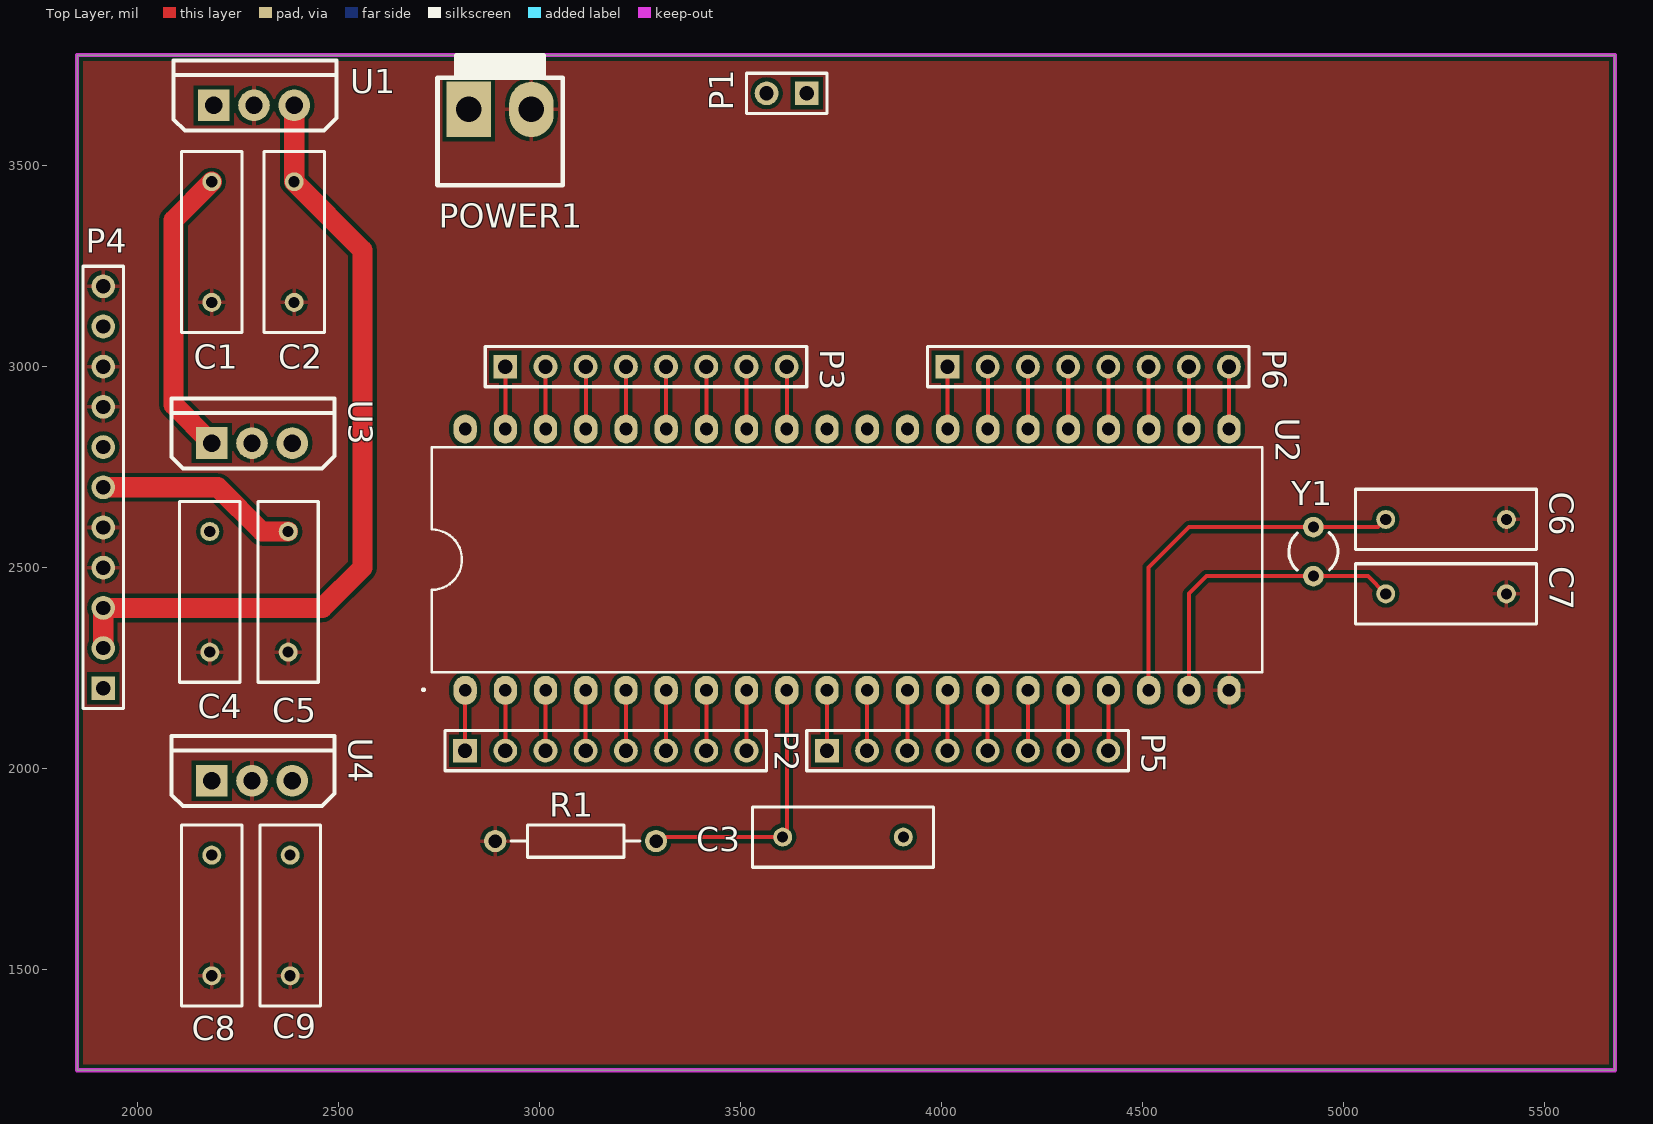
[diagram p0: Top Layer view]
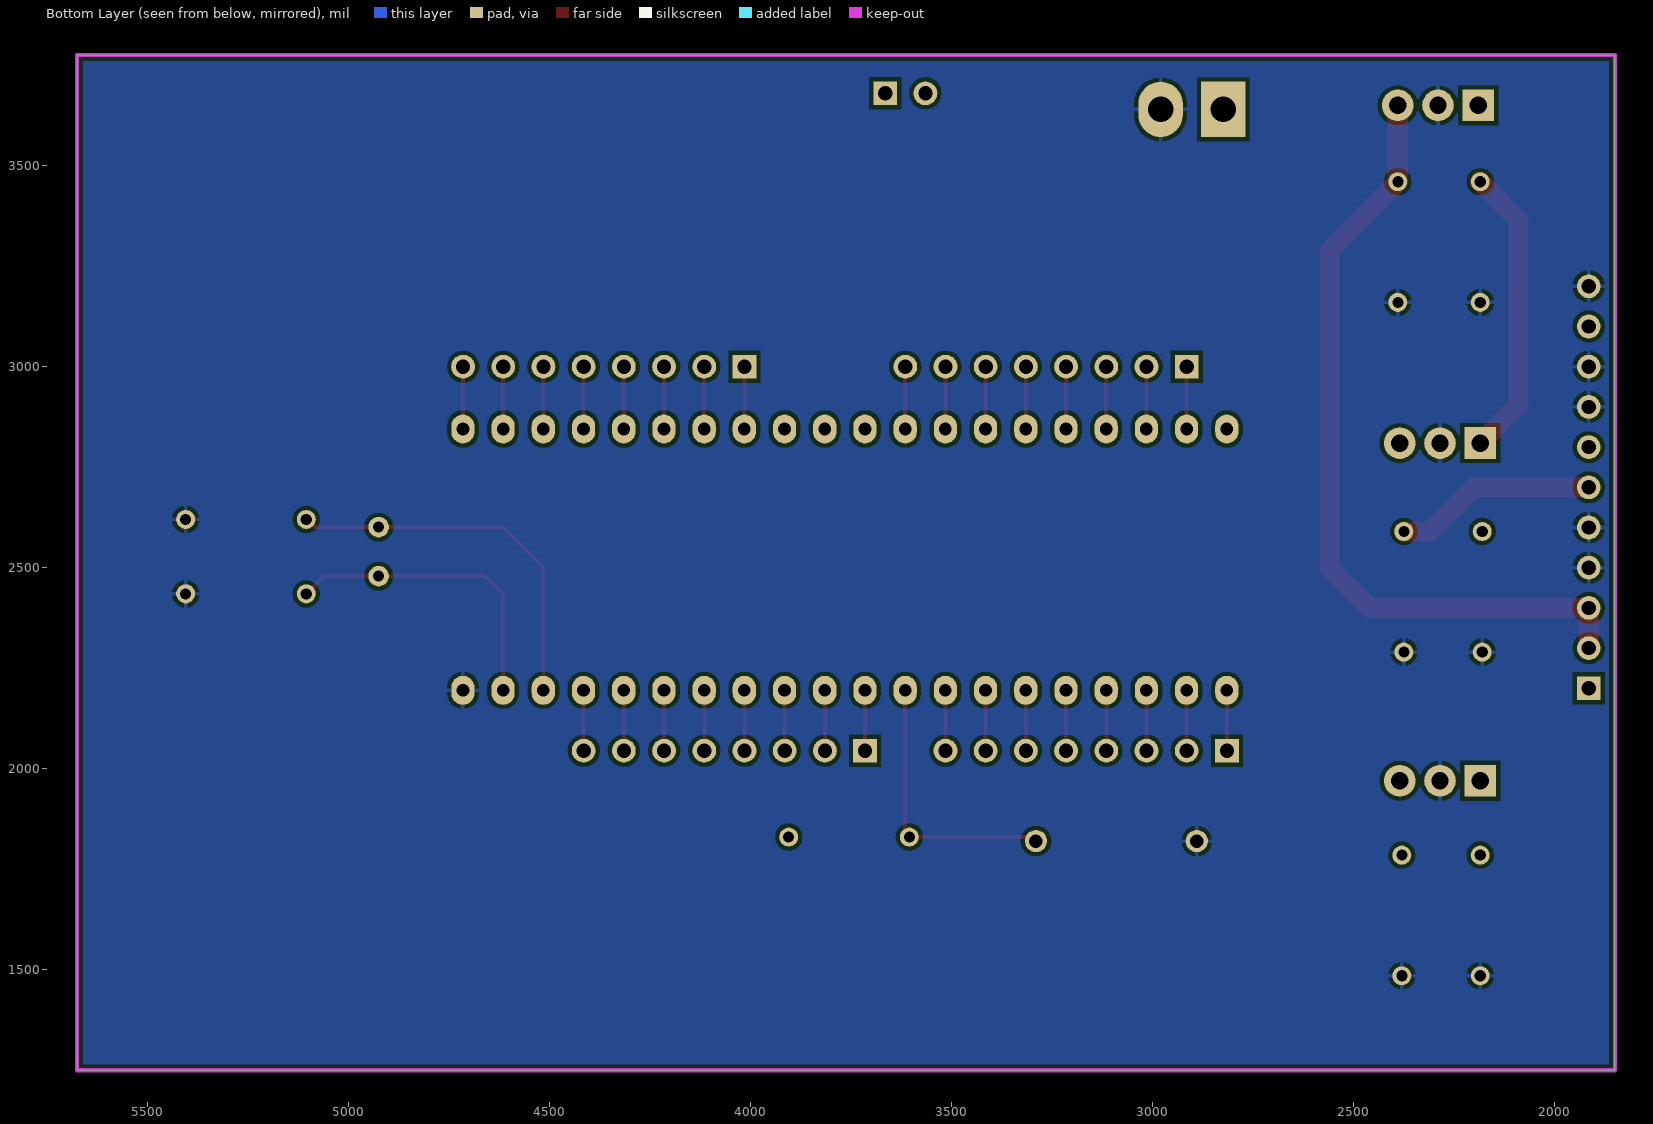
[diagram p1: Bottom Layer view, seen from below]
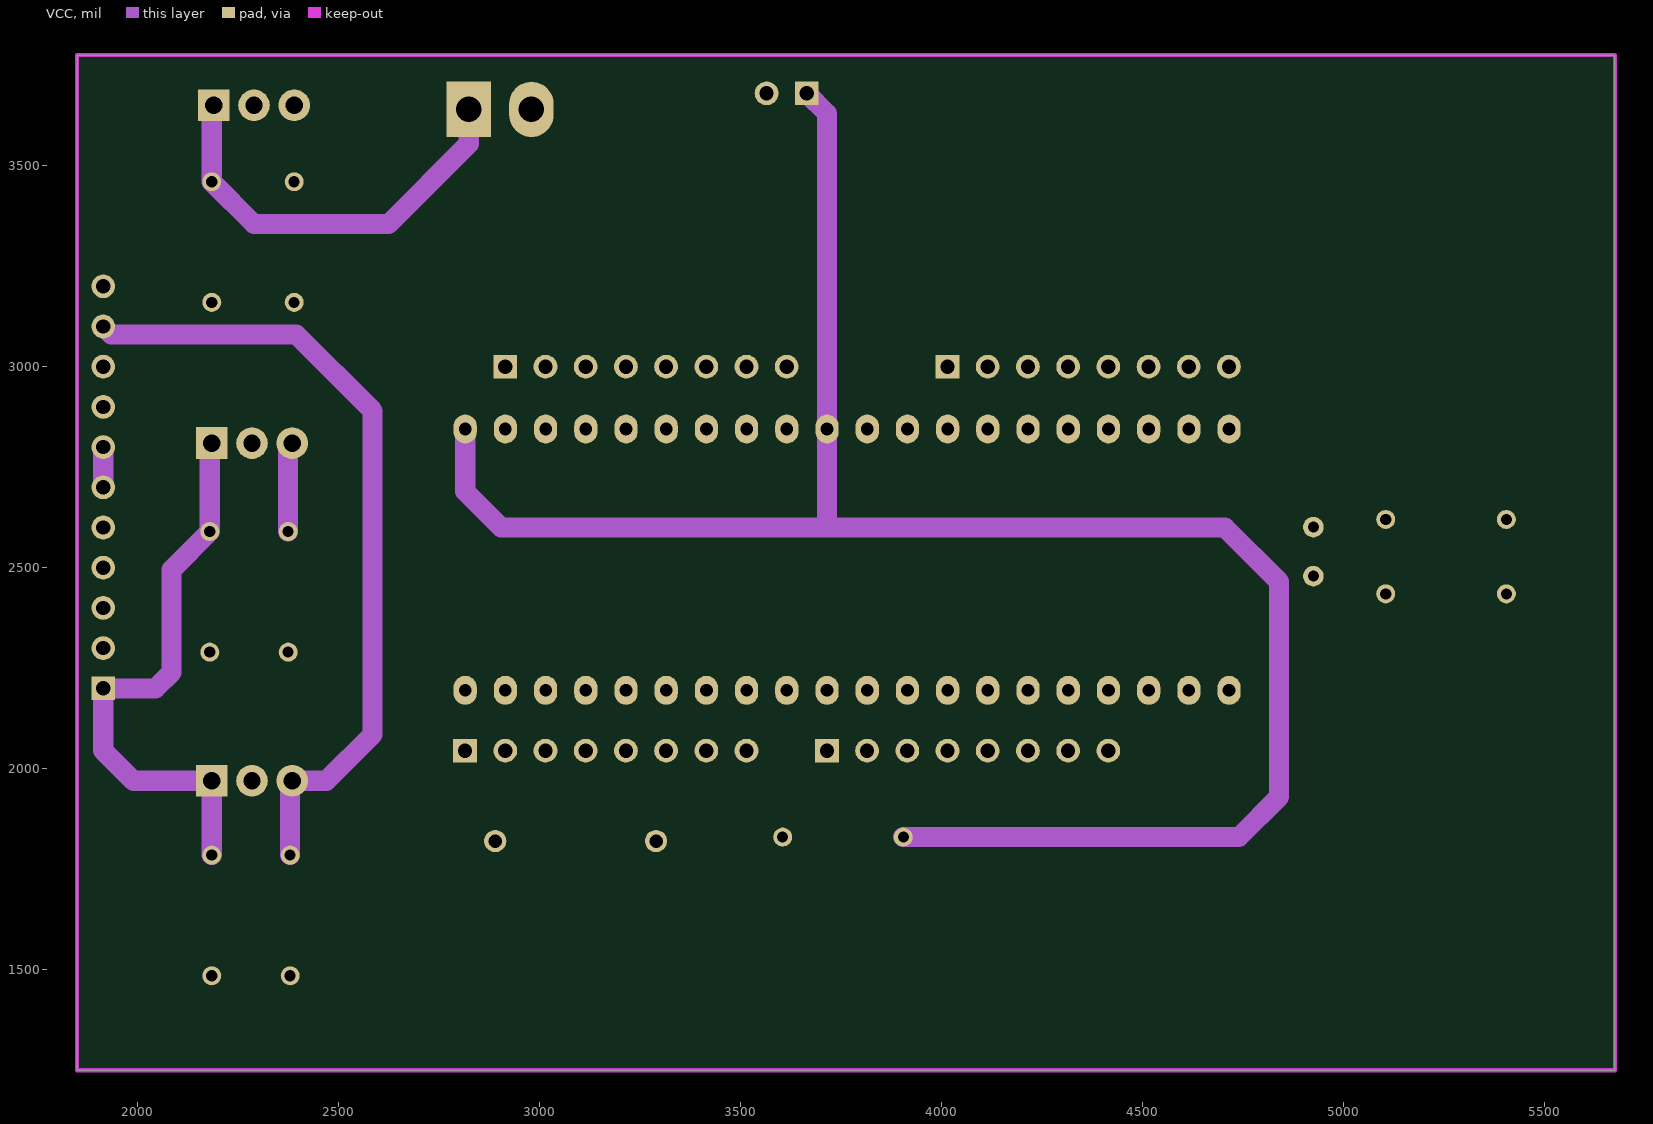
[diagram p2: VCC]
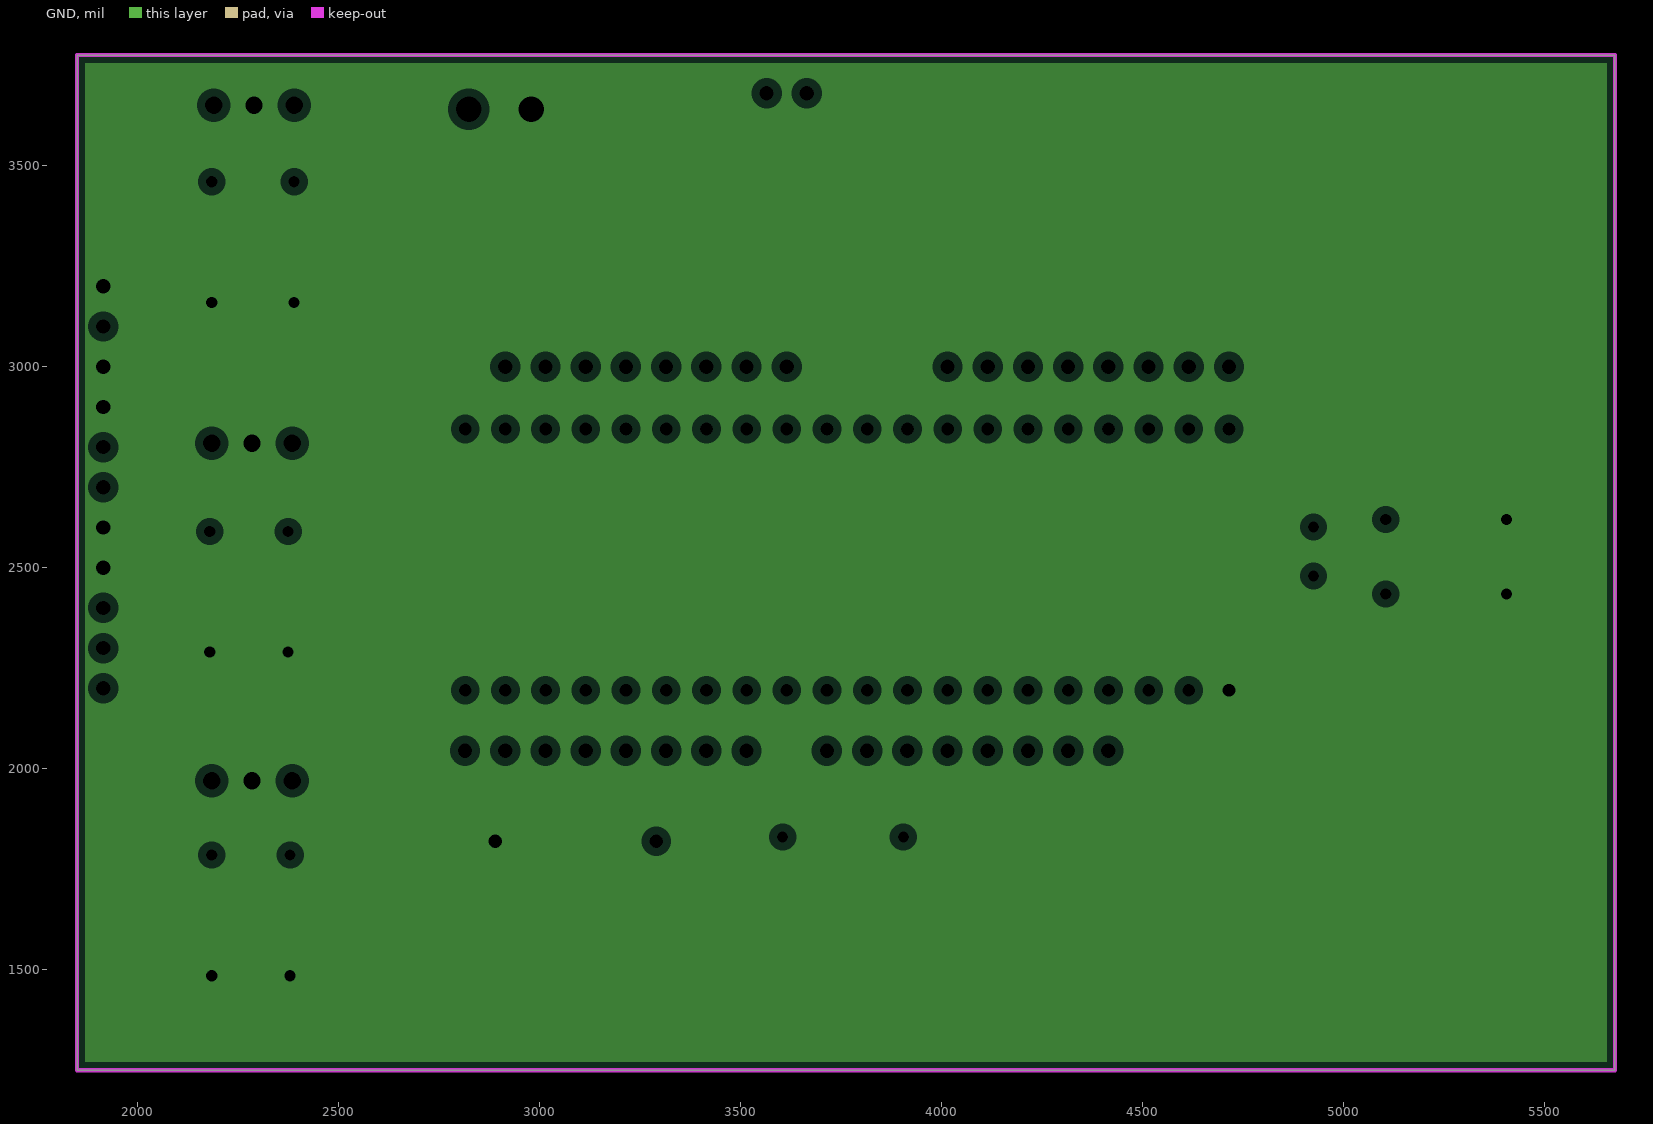
[diagram p3: GND, clearances drawn from the general rule]
# Altium PCB MISC82800.PcbDoc
Units mil, origin at the board's own origin, x right, y up, seen from the top; angles counter-clockwise.
Board outline 3825 x 2525 mil, 4 copper layers (Top Layer, VCC, GND, Bottom Layer), stack 30.634 mil thick; 22 components, 41 nets, 118 pads, 0 vias.

## Layer stack, top to bottom
Top Solder: solder mask 0.4, Solder Resist, Dk 3.5
Top Layer: signal copper 1.4
Dielectric 1: core 10, FR-4, Dk 4.2
VCC: signal copper 1.417
Dielectric 3: prepreg 5, Dk 4.2
GND: plane copper 1.417, net GND
Dielectric 2: core 10, Dk 4.2
Bottom Layer: signal copper 1.4
Bottom Solder: solder mask 0.4, Solder Resist, Dk 3.5

## Board outline
1850,1250 5675,1250 5675,3775 1850,3775

## Design rules (kind name [scope] priority, off if disabled: settings)
Clearance [All] p1: gap=10
MinimumSolderMaskSliver [All] p1: minsoldermaskwidth=0
PlaneClearance [All] p1: clearance=20
PlaneConnect [All] p1: planeconnectstyle=Relief reliefexpansion=20 reliefentries=4 reliefconductorwidth=10 reliefairgap=10
PolygonConnect [All] p1: connectstyle=Relief reliefconductorwidth=10 reliefentries=4 polygonreliefangle="90 Angle" airgapwidth=10
RoutingVias [All] p1: holewidth=28 width=50 viastyle="Through Hole" minholewidth=28 minwidth=50 maxholewidth=28 maxwidth=50
SilkToSilkClearance [All] p1: silktosilkclearance=0
SilkToSolderMaskClearance [IsPad] p1: minsilkscreentomaskgap=0 clearancetoexposedcopper=TRUE
SolderMaskExpansion [All] p1: expansion=4
Width [All] p1: maxlimit=50 minlimit=10 preferedwidth=10
25 further rules are at their usual default settings.

## Components (designator, comment, footprint, x,y, rotation, side; value= is the part's Value field where it differs from the comment)
C1 "0.33UF" RAD-0.3 2185,3310 r270 top
C2 "0.1UF" RAD-0.3 2390,3310 r270 top
C3 "10UF" RAD-0.3 3755,1830 r180 top
C4 "0.33UF" RAD-0.3 2180,2440 r270 top
C5 "0.1UF" RAD-0.3 2375,2440 r270 top
C6 "22pF" RAD-0.3 5255,2620 r0 top
C7 "22pF" RAD-0.3 5255,2435 r0 top
C8 "0.33UF" RAD-0.3 2185,1635 r270 top
C9 "0.1UF" RAD-0.3 2380,1635 r270 top
P1 "Header 2" HDR1X2 3665,3680 r180 top
P2 "Header 8" HDR1X8 2815,2045 r0 top
P3 "Header 8" HDR1X8 2915,3000 r0 top
P4 "Header 11" HDR1X11 1915,2200 r90 top
P5 "Header 8" HDR1X8 3715,2045 r0 top
P6 "Header 8" HDR1X8 4015,3000 r0 top
POWER1 "Terminal block" VH3.96-2A 2824.09,3640 r0 top
R1 "10K" AXIAL-0.4 3090,1820 r0 top
U1 "LM7805" TO220A 2290,3650 r0 top
U2 "STC89C52RC" STC89C52RC 3755,2520 r0 top
U3 "LM7805" TO220A 2285,2810 r0 top
U4 "LM7806" TO220A 2285,1970 r0 top
Y1 "XTAL" R38 4925,2540 r180 top

## Footprints (in the part's own frame and the unit in brackets; to place one, negate y for a bottom-side part, rotate by r counter-clockwise, add the part's x,y. Pads: shape width x height; smd on the part's side, far side on the other; paste and mask are expansions set on the pad)
AXIAL-0.4 [mm] "Axial Device, Thru-Hole; 2 Leads; 0.4 in Pin Spacing"
  round 1.4 hole 0.85: 1(-5.08,0) 2(5.08,0)
  silkscreen extent -4.06,-1.02 4.06,1.02
HDR1X2 [mm] "Connector; Header; 2 Position"
  rect 1.5x1.5 hole 0.9: 1(0,0)
  round 1.5 hole 0.9: 2(2.54,0)
  silkscreen extent -1.27,-1.27 3.81,1.27
HDR1X8 [mm] "Connector; Header; 8 Position"
  rect 1.5x1.5 hole 0.9: 1(0,0)
  round 1.5 hole 0.9: 2(2.54,0) 3(5.08,0) 4(7.62,0) 5(10.16,0) 6(12.7,0) 7(15.24,0) 8(17.78,0)
  silkscreen extent -1.27,-1.27 19.05,1.27
HDR1X11 [mm] "Connector; Header; 11 Position"
  rect 1.5x1.5 hole 0.9: 1(0,0)
  round 1.5 hole 0.9: 2(2.54,0) 3(5.08,0) 4(7.62,0) 5(10.16,0) 6(12.7,0) 7(15.24,0) 8(17.78,0) 9(20.32,0) 10(22.86,0) 11(25.4,0)
  silkscreen extent -1.27,-1.27 26.67,1.27
R38 [mm] "Crystal, Thru-Hole; 2 Leads; Body 3.1 x 8.2 mm (Dia.xH)"
  round 1.3 hole 0.7: 1(0,1.55) 2(0,-1.55)
  silkscreen extent -1.55,-1.19 1.55,1.17
RAD-0.3 [mm] "Radial Cap, Thru-Hole; 2 Leads; 0.3 in Pin Spacing"
  round 1.2 hole 0.7: 1(-3.81,0) 2(3.81,0)
  silkscreen extent -5.71,-1.91 5.71,1.91
STC89C52RC [mm]
  oval 1.467x1.833 hole 0.8 paste+0 mask+0.051: 1(-23.868,-8.255) 2(-21.328,-8.255) 3(-18.788,-8.255) 4(-16.248,-8.255) 5(-13.708,-8.255) 6(-11.168,-8.255) 7(-8.628,-8.255) 8(-6.088,-8.255) 9(-3.548,-8.255) 10(-1.008,-8.255) 11(1.532,-8.255) 12(4.072,-8.255) 13(6.612,-8.255) 14(9.152,-8.255) 15(11.692,-8.255) 16(14.232,-8.255) 17(16.772,-8.255) 18(19.312,-8.255) 19(21.852,-8.255) 20(24.392,-8.255) 21(24.392,8.255) 22(21.852,8.255) 23(19.312,8.255) 24(16.772,8.255) 25(14.232,8.255) 26(11.692,8.255) 27(9.152,8.255) 28(6.612,8.255) 29(4.072,8.255) 30(1.532,8.255) 31(-1.008,8.255) 32(-3.548,8.255) 33(-6.088,8.255) 34(-8.628,8.255) 35(-11.168,8.255) 36(-13.708,8.255) 37(-16.248,8.255) 38(-18.788,8.255) 39(-21.328,8.255) 40(-23.868,8.255)
  silkscreen extent -26.58,-8.3 26.5,7.11
TO220A [mm] "220，3脚晶体管"
  rect 2x2 hole 1.1: 1(-2.54,0)
  round 2 hole 1.1: 2(0,0) 3(2.54,0)
  silkscreen extent -5.08,-1.6 5.21,2.82, body extent -5.08,-1.45 5.22,2.98, height 18.5
VH3.96-2A [mm]
  rect 2.8x3.5 hole 1.6: 1(0,0)
  oval 2.8x3.5 hole 1.6: 2(3.96,0)
  silkscreen extent -1.98,-4.8 5.94,3.4, body extent -1.98,-4.8 5.94,3.6, height 14.6

## Part data
C1 C2 C3 C4 C5 C6 C7 C8 C9: library part Cap, "Capacitor"
P1: "Header, 2-Pin"
P2 P3 P5 P6: "Header, 8-Pin"
P4: "Header, 11-Pin"
POWER1: library part VH2
R1: library part Res2, "Resistor"
U4: library part LM7805
Y1: "Crystal Oscillator"

## Nets (pads, with @x,y where several pads share a name; then routed paths per layer and width w, separated by ;. In a path a pad name is that pad's centre, name@x,y a point inside that pad or via, vN(x,y) a via of type N, cw(c..) or ccw(c..) an arc to the next point about the centre after c; other vN are vias at no path point)
5V1: C2.1 P4.2 P4.3 U1.3 | length 2006.8
  Top Layer w50: P4.2 P4.3 2460,2400 2560,2500 2560,3290 C2.1 U1.3
5V2: C5.1 P4.6 P4.7 U3.3 | length 829.7
  Top Layer w50: P4.6 2200,2700 2310,2590 C5.1
  VCC w50: P4.6 P4.7 ; C5.1 2375,2800 U3.3
6V: C9.1 P4.10 U4.3 | length 1996.7
  VCC w50: P4.10 1935,3080 2395,3080 2585,2890 2585,2085 2470,1970 U4.3 2380,1965 C9.1
GND: C1.2 C2.2 C4.2 C5.2 C6.2 C7.2 C8.2 C9.2 P4.4 P4.5 P4.8 P4.9 P4.11 POWER1.2 R1.1 U1.2 U2.20 U3.2 U4.2
NetC1_1: C1.1 C4.1 C8.1 P4.1 POWER1.1 U1.1 U3.1 U4.1 | length 3210.8
  Top Layer w50: U3.1 2090,2905 2090,3365 C1.1
  VCC w50: C8.1 U4.1 1990,1970 1915,2045 P4.1 2045,2200 2085,2240 2085,2495 C4.1 2180,2805 U3.1 ; U1.1 2185,3645 C1.1 2290,3355 2625,3355 2824.09,3554.09 POWER1.1
NetC3_2: C3.2 R1.2 U2.9 | length 688.4
  Top Layer w10: R1.2 3300,1830 C3.2 3615.33,1840.33 U2.9
NetC6_1: C6.1 U2.18 Y1.2 | length 944.6
  Top Layer w10: U2.18 4515.33,2500.33 4616.02,2601.02 Y1.2 5086.02,2601.02 C6.1
NetC7_1: C7.1 U2.19 Y1.1 | length 766.3
  Top Layer w10: U2.19 4615.33,2435.33 4658.98,2478.98 Y1.1 5061.02,2478.98 C7.1
NetP2_1: P2.1 U2.1 | length 150.1
  Top Layer w10: P2.1 2815.33,2045.33 U2.1
NetP2_2: P2.2 U2.2 | length 150.1
  Top Layer w10: P2.2 2915,2194.67 U2.2
NetP2_3: P2.3 U2.3 | length 150.1
  Top Layer w10: P2.3 3015,2194.67 U2.3
NetP2_4: P2.4 U2.4 | length 150.1
  Top Layer w10: P2.4 3115,2194.67 U2.4
NetP2_5: P2.5 U2.5 | length 150.1
  Top Layer w10: P2.5 3215,2194.67 U2.5
NetP2_6: P2.6 U2.6 | length 150.1
  Top Layer w10: P2.6 3315,2194.67 U2.6
NetP2_7: P2.7 U2.7 | length 150.1
  Top Layer w10: P2.7 3415,2194.67 U2.7
NetP2_8: P2.8 U2.8 | length 150.1
  Top Layer w10: P2.8 3515,2194.67 U2.8
NetP3_1: P3.1 U2.39 | length 155.1
  Top Layer w10: P3.1 2915.33,2999.67 U2.39
NetP3_2: P3.2 U2.38 | length 155.1
  Top Layer w10: P3.2 3015.33,2999.67 U2.38
NetP3_3: P3.3 U2.37 | length 155.1
  Top Layer w10: P3.3 3115.33,2999.67 U2.37
NetP3_4: P3.4 U2.36 | length 155.1
  Top Layer w10: P3.4 3215.33,2999.67 U2.36
NetP3_5: P3.5 U2.35 | length 155.1
  Top Layer w10: P3.5 3315.33,2999.67 U2.35
NetP3_6: P3.6 U2.34 | length 155.1
  Top Layer w10: P3.6 3415.33,2999.67 U2.34
NetP3_7: P3.7 U2.33 | length 155.1
  Top Layer w10: P3.7 3515.33,2999.67 U2.33
NetP3_8: P3.8 U2.32 | length 155.1
  Top Layer w10: P3.8 3615.33,2999.67 U2.32
NetP5_1: P5.1 U2.10 | length 150.1
  Top Layer w10: P5.1 3715,2194.67 U2.10
NetP5_2: P5.2 U2.11 | length 150.1
  Top Layer w10: P5.2 3815,2194.67 U2.11
NetP5_3: P5.3 U2.12 | length 150.1
  Top Layer w10: P5.3 3915,2194.67 U2.12
NetP5_4: P5.4 U2.13 | length 150.1
  Top Layer w10: P5.4 4015,2194.67 U2.13
NetP5_5: P5.5 U2.14 | length 150.1
  Top Layer w10: P5.5 4115,2194.67 U2.14
NetP5_6: P5.6 U2.15 | length 150.1
  Top Layer w10: P5.6 4215,2194.67 U2.15
NetP5_7: P5.7 U2.16 | length 150.1
  Top Layer w10: P5.7 4315,2194.67 U2.16
NetP5_8: P5.8 U2.17 | length 150.1
  Top Layer w10: P5.8 4415,2194.67 U2.17
NetP6_1: P6.1 U2.28 | length 155.1
  Top Layer w10: P6.1 4015.33,2999.67 U2.28
NetP6_2: P6.2 U2.27 | length 155.1
  Top Layer w10: P6.2 4115.33,2999.67 U2.27
NetP6_3: P6.3 U2.26 | length 155.1
  Top Layer w10: P6.3 4215.33,2999.67 U2.26
NetP6_4: P6.4 U2.25 | length 155.1
  Top Layer w10: P6.4 4315.33,2999.67 U2.25
NetP6_5: P6.5 U2.24 | length 155.1
  Top Layer w10: P6.5 4415.33,2999.67 U2.24
NetP6_6: P6.6 U2.23 | length 155.1
  Top Layer w10: P6.6 4515.33,2999.67 U2.23
NetP6_7: P6.7 U2.22 | length 155.1
  Top Layer w10: P6.7 4615.33,2999.67 U2.22
NetP6_8: P6.8 U2.21 | length 155.1
  Top Layer w10: P6.8 4715.33,2999.67 U2.21
VCC: C3.1 P1.1 U2.31 U2.40 | length 4887.5
  VCC w50: U2.40 2815.33,2689.67 2905,2600 3710,2600 ; P1.1 3715.33,3629.67 U2.31 3715.33,2605.33 3710,2600 ; C3.1 4740,1830 4840,1930 4840,2465 4705,2600 3710,2600
pads on no net: P1.2 U2.29 U2.30

## Polygon pours and split planes (outlines as drawn)
GND on Top Layer "D" (solid, remove dead copper, pour order 0): 1470,3880 5955,3880 6110,4035 5885,3810 5885,1170 1625,1170 1585,1130
GND on Bottom Layer "D" (solid, remove dead copper, pour order 2): 1340,3940 1490,3790 6395,3790 6395,1795 5765,1165 5650,1050 1305,1050
GND on GND (split plane): 5654.9,1270.1 1870.1,1270.1 1870.1,3754.9 5654.9,3754.9

## Keep-outs
Keep-Out Layer:
  lines w10: 1850,1250 5675,1250 5675,1330 5675,3775 1850,3775 1850,1250